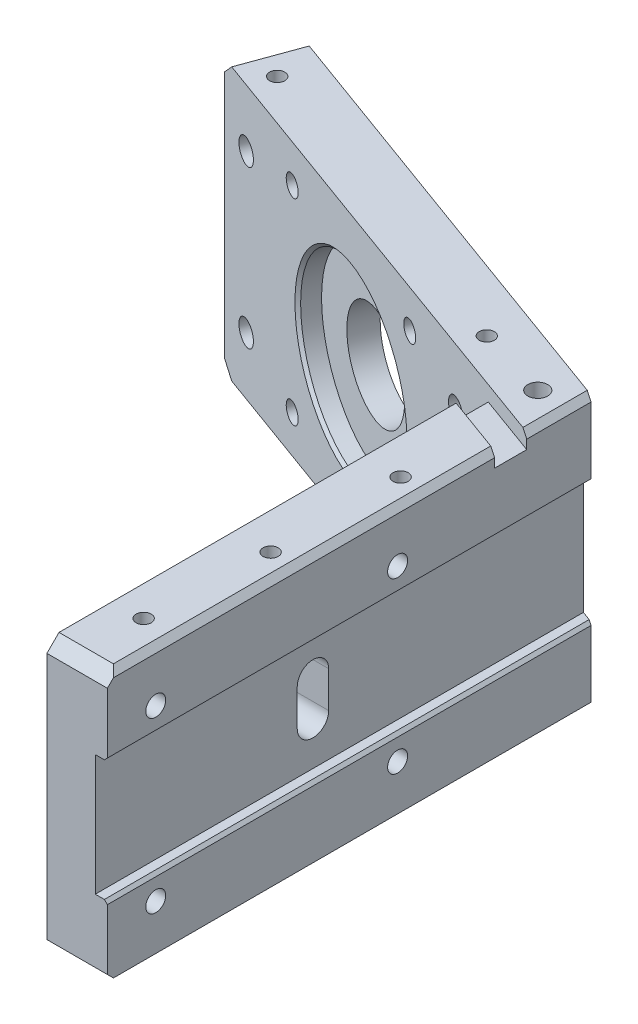
from build123d import *

# Parameters (mm, degrees)
BOSS_EXTRUDE1_DEPTH        = 45
SKETCH2_R                  = 8
CUT_EXTRUDE1_DEPTH         = 36
SKETCH3_R                  = 15
CUT_EXTRUDE2_DEPTH         = 3.2
SKETCH4_R                  = 2
CUT_EXTRUDE3_DEPTH         = 25
SKETCH5_R                  = 4
CUT_EXTRUDE4_DEPTH         = 2
SKETCH7_R                  = 1
CUT_EXTRUDE5_DEPTH         = 8
M3_TAPPED_HOLE1_AT_2_COUNT = 2
M3_TAPPED_HOLE1_AT_2_PITCH = 58
SKETCH13_R                 = 17.5
CUT_EXTRUDE8_DEPTH         = 2.5
CUT_EXTRUDE9_DEPTH         = 2.5
M4_TAPPED_HOLE2_D          = 3.3
M4_TAPPED_HOLE2_DEPTH      = 10.1
M4_TAPPED_HOLE2_TIP        = 0.991420021
CHAMFER1_SIZE              = 2
M4_TAPPED_HOLE3_D          = 3.3
M4_TAPPED_HOLE3_DEPTH      = 10.1
M4_TAPPED_HOLE3_TIP        = 0.991420021
M3_TAPPED_HOLE2_D          = 2.5
M3_TAPPED_HOLE2_DEPTH      = 7.5
M3_TAPPED_HOLE2_TIP        = 0.751075774
SKETCH9_W                  = 82.200084453
SKETCH9_H                  = 20
CUT_EXTRUDE10_DEPTH        = 2
CUT_EXTRUDE11_DEPTH        = 140.349930982
CHAMFER2_SIZE              = 1
CHAMFER3_SIZE              = 0.5
M4_TAPPED_HOLE4_D          = 3.3
CIRPATTERN1_COUNT          = 4
CHAMFER4_SIZE              = 0.5


with BuildPart() as part:
    # Sketch1 → Boss-Extrude1 (new body)
    with BuildSketch(Plane(origin=(0, 0, 0), x_dir=(1, 0, 0), z_dir=(0, 1, 0))):
        Polygon((-75.175409663, 107.361611466), (0, 80), (0, 0), (-10, 0), (-10, 72.997924618), (-78.595611096, 97.964685258), align=None)
    extrude(amount=BOSS_EXTRUDE1_DEPTH)

    # Sketch2 → Cut-Extrude1 (cut)
    with BuildSketch(Plane(origin=(25.711504387, 0, -70.641777725), x_dir=(-0.9396926207859106, 0, -0.3420201433256628), z_dir=(0.3420201433256628, 0, -0.9396926207859106))):
        with Locations((72.361611466, 22.5)):
            Circle(SKETCH2_R)
    extrude(amount=-CUT_EXTRUDE1_DEPTH, mode=Mode.SUBTRACT)

    # Sketch3 → Cut-Extrude2 (cut)
    with BuildSketch(Plane(origin=(22.291302954, 0, -61.244851517), x_dir=(0.9396926207859108, 0, 0.34202014332566244), z_dir=(-0.34202014332566244, 0, 0.9396926207859108))):
        with Locations((-72.361611466, 22.5)):
            Circle(SKETCH3_R)
    extrude(amount=-CUT_EXTRUDE2_DEPTH, mode=Mode.SUBTRACT)

    # Sketch4 → Cut-Extrude3 (cut)
    with BuildSketch(Plane(origin=(25.711504387, 0, -70.641777725), x_dir=(-0.9396926207859106, 0, -0.3420201433256628), z_dir=(0.3420201433256628, 0, -0.9396926207859106))):
        with Locations((43.361611466, 35.5)):
            Circle(SKETCH4_R)
        with Locations((101.361611466, 35.5)):
            Circle(SKETCH4_R)
        with Locations((101.361611466, 9.5)):
            Circle(SKETCH4_R)
        with Locations((43.361611466, 9.5)):
            Circle(SKETCH4_R)
    extrude(amount=-CUT_EXTRUDE3_DEPTH, mode=Mode.SUBTRACT)

    # Sketch5 → Cut-Extrude4 (cut)
    with BuildSketch(Plane(origin=(25.711504387, 0, -70.641777725), x_dir=(-0.9396926207859106, 0, -0.3420201433256628), z_dir=(0.3420201433256628, 0, -0.9396926207859106))):
        with Locations((43.361611466, 35.5)):
            Circle(SKETCH5_R)
        with Locations((43.361611466, 9.5)):
            Circle(SKETCH5_R)
        with Locations((101.361611466, 9.5)):
            Circle(SKETCH5_R)
        with Locations((101.361611466, 35.5)):
            Circle(SKETCH5_R)
    extrude(amount=-CUT_EXTRUDE4_DEPTH, mode=Mode.SUBTRACT)

    # Sketch7 → Cut-Extrude5 (cut)
    with BuildSketch(Plane.XZ):
        with Locations(Location((-71.589374798, -99.671334881, 0), (0, 0, 270))):
            Circle(SKETCH7_R)
        with Locations(Location((-17.087202793, -79.834166568, 0), (0, 0, 270))):
            Circle(SKETCH7_R)
    extrude(amount=-CUT_EXTRUDE5_DEPTH, mode=Mode.SUBTRACT)

    # Sketch8 → M3 Tapped Hole1 (revolve, cut)
    with BuildSketch(Plane(origin=(-17.087202793, 0, -79.834166568), x_dir=(0, 0, -1), z_dir=(1, 0, 0))):
        Polygon((0, 0), (0, 10.251075774), (1.25, 9.5), (1.25, 0), align=None)
    m3_tapped_hole1 = revolve(axis=Axis((-17.087202793, -6.35, -79.834166568), (0, 1, 0)), mode=Mode.SUBTRACT)

    # M3 Tapped Hole1 at 2: M3 Tapped Hole1 ×2
    with Locations(*[Vector(-0.9396926207859108, 0, -0.3420201433256624) * (i * M3_TAPPED_HOLE1_AT_2_PITCH) for i in range(1, M3_TAPPED_HOLE1_AT_2_COUNT)]):
        add(m3_tapped_hole1, mode=Mode.SUBTRACT)

    # Mirror1: M3 Tapped Hole1 across plane
    add(m3_tapped_hole1.mirror(Plane(origin=(0, 22.5, 0), x_dir=(0, 0, 1), z_dir=(0, -1, 0))), mode=Mode.SUBTRACT)

    # Mirror1 copy 1 sketch → Mirror1 copy 1 (revolve, cut)
    with BuildSketch(Plane(origin=(-71.589374798, 45, -99.671334881), x_dir=(0, 0, -1), z_dir=(1, 0, 0))):
        Polygon((0, 0), (0, -10.251075774), (1.25, -9.5), (1.25, 0), align=None)
    revolve(axis=Axis((-71.589374798, 51.35, -99.671334881), (0, 1, 0)), mode=Mode.SUBTRACT)

    # Sketch13 → Cut-Extrude8 (cut)
    with BuildSketch(Plane(origin=(25.711504387, 0, -70.641777725), x_dir=(-0.9396926207859106, 0, -0.3420201433256628), z_dir=(0.34202014332566283, 0, -0.9396926207859106))):
        with Locations((72.361611466, 22.5)):
            Circle(SKETCH13_R)
    extrude(amount=-CUT_EXTRUDE8_DEPTH, mode=Mode.SUBTRACT)

    # Sketch15 → Cut-Extrude9 (cut)
    with BuildSketch(Plane(origin=(0, 45, 0), x_dir=(1, 0, 0), z_dir=(0, 1, 0))):
        Polygon((-10, 72.997924618), (1.8, 68.703075854), (1.8, 63.382186991), (-10, 67.677035756), align=None)
    extrude(amount=-CUT_EXTRUDE9_DEPTH, mode=Mode.SUBTRACT)

    # M4 Tapped Hole2
    with Locations(Plane(origin=(-5.084529925, 45, -76.263684243), x_dir=(0, 0, 1), z_dir=(0, 1, 0))):
        with Locations((0, 0)):
            Hole(M4_TAPPED_HOLE2_D / 2, depth=M4_TAPPED_HOLE2_DEPTH)
            with Locations((0, 0, -(M4_TAPPED_HOLE2_DEPTH + M4_TAPPED_HOLE2_TIP / 2))):  # 118° drill point
                Cone(0, M4_TAPPED_HOLE2_D / 2, M4_TAPPED_HOLE2_TIP, mode=Mode.SUBTRACT)

    # Chamfer1
    chamfer1_edges = [part.edges().sort_by_distance(p)[0] for p in [
        (-76.88551038, 45, -102.663148362),
        (-5, 45, 0),
        (-5, 0, 0),
        (-76.88551038, 0, -102.663148362),
    ]]
    chamfer(chamfer1_edges, length=CHAMFER1_SIZE)

    # M4 Tapped Hole3
    with Locations(Plane(origin=(0, 0, 0), x_dir=(0, 0, -1), z_dir=(1, 0, 0))):
        with Locations((48, 36.5), (48, 8.5), (8, 8.5), (8, 36.5)):
            Hole(M4_TAPPED_HOLE3_D / 2, depth=M4_TAPPED_HOLE3_DEPTH)
            with Locations((0, 0, -(M4_TAPPED_HOLE3_DEPTH + M4_TAPPED_HOLE3_TIP / 2))):  # 118° drill point
                Cone(0, M4_TAPPED_HOLE3_D / 2, M4_TAPPED_HOLE3_TIP, mode=Mode.SUBTRACT)

    # M3 Tapped Hole2
    with Locations(Plane(origin=(0, 45, 0), x_dir=(1, 0, 0), z_dir=(0, 1, 0))):
        with Locations((-4, 52.5), (-4, 31)):
            Hole(M3_TAPPED_HOLE2_D / 2, depth=M3_TAPPED_HOLE2_DEPTH)
            with Locations((0, 0, -(M3_TAPPED_HOLE2_DEPTH + M3_TAPPED_HOLE2_TIP / 2))):  # 118° drill point
                Cone(0, M3_TAPPED_HOLE2_D / 2, M3_TAPPED_HOLE2_TIP, mode=Mode.SUBTRACT)

    # Sketch23 → M3 Tapped Hole4 (revolve, cut)
    with BuildSketch(Plane(origin=(-5, 0, -11), x_dir=(0, 0, -1), z_dir=(1, 0, 0))):
        Polygon((0, 0), (0, 8.251075774), (1.25, 7.5), (1.25, 0), align=None)
    m3_tapped_hole4 = revolve(axis=Axis((-5, -6.35, -11), (0, 1, 0)), mode=Mode.SUBTRACT)

    # Mirror2: M3 Tapped Hole4 across plane
    add(m3_tapped_hole4.mirror(Plane(origin=(0, 22.5, 0), x_dir=(0, 0, 1), z_dir=(0, -1, 0))), mode=Mode.SUBTRACT)

    # Sketch9 → Cut-Extrude10 (cut)
    with BuildSketch(Plane(origin=(0, 0, 0), x_dir=(0, 0, -1), z_dir=(1, 0, 0))):
        with Locations((41.100042227, 22.5)):
            Rectangle(SKETCH9_W, SKETCH9_H)
    extrude(amount=-CUT_EXTRUDE10_DEPTH, mode=Mode.SUBTRACT)

    # Sketch25 → Cut-Extrude11 (cut, through all)
    with BuildSketch(Plane(origin=(-2, 0, 0), x_dir=(0, 0, -1), z_dir=(1, 0, 0))):
        with BuildLine():
            Line((38.6, 25.5), (38.6, 19.5))
            ThreePointArc((38.6, 19.5), (36, 16.9), (33.4, 19.5))
            Line((33.4, 19.5), (33.4, 25.5))
            ThreePointArc((33.4, 25.5), (36, 28.1), (38.6, 25.5))
        make_face()
    extrude(amount=-CUT_EXTRUDE11_DEPTH, mode=Mode.SUBTRACT)

    # Chamfer2
    chamfer2_edges = [part.edges().sort_by_distance(p)[0] for p in [
        (0, 45, -74.679111138),
        (0, 45, -33.018666706),
        (0, 0, -41),
    ]]
    chamfer(chamfer2_edges, length=CHAMFER2_SIZE)

    # Chamfer3
    chamfer3_edges = [part.edges().sort_by_distance(p)[0] for p in [
        (-59.80175868, 22.5, -91.124282392),
    ]]
    chamfer(chamfer3_edges, length=CHAMFER3_SIZE)

    # M4 Tapped Hole4 (through all)
    with Locations(Plane(origin=(22.291302954, 0, -61.244851517), x_dir=(0.9396926207859106, 0, 0.34202014332566244), z_dir=(-0.34202014332566244, 0, 0.9396926207859106))):
        with Locations((-88.625067433, 38.763455967)):
            m4_tapped_hole4 = Hole(M4_TAPPED_HOLE4_D / 2)

    # CirPattern1: M4 Tapped Hole4 ×4 about axis
    cirpattern1_axis = Axis((-67.997672323, 22.5, -24.749128725), (-0.34202014332566244, 0, 0.9396926207859106))
    for i in range(1, CIRPATTERN1_COUNT):
        add(m4_tapped_hole4.rotate(cirpattern1_axis, i * 360 / CIRPATTERN1_COUNT), mode=Mode.SUBTRACT)

    # Chamfer4
    chamfer4_edges = [part.edges().sort_by_distance(p)[0] for p in [
        (0, 12.5, -40),
        (0, 32.5, -40),
    ]]
    chamfer(chamfer4_edges, length=CHAMFER4_SIZE)


solid = part.part
